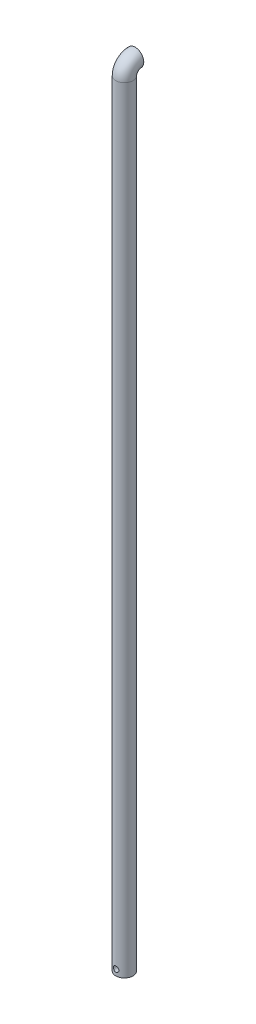
from build123d import *

# Parameters (mm, degrees)
SKETCH1_R               = 8
SKETCH1_R_2             = 3
SKETCH3_R               = 3
BOSS_EXTRUDE1_DEPTH     = 3
CUT_EXTRUDE2_DEPTH      = 731.265705073
CUT_EXTRUDE2_DEPTH_BACK = 731.265705073
SKETCH4_R               = 2.5


with BuildPart() as part:
    # Sweep1: sweep along a path in Sketch2
    with BuildLine(Plane(origin=(0, 0, 0), x_dir=(0, 0, -1), z_dir=(1, 0, 0))) as sweep1_path:
        Line((0, 0), (-0.05, 0))
        ThreePointArc((-0.05, 0), (-7.085712473, -2.914287527), (-10, -9.95))
        Line((-10, -9.95), (-10, -730))
    # Sketch1 → Sweep1 (sweep)
    with BuildSketch(Plane.XY):
        Circle(SKETCH1_R)
        Circle(SKETCH1_R_2, mode=Mode.SUBTRACT)
    sweep(path=sweep1_path.line)

    # Sketch3 → Boss-Extrude1 (add)
    with BuildSketch(Plane.XZ.offset(730)):
        with Locations(Location((0, 10, 0), (0, 0, 270))):
            Circle(SKETCH3_R)
    extrude(amount=-BOSS_EXTRUDE1_DEPTH)

    # Sketch4 → Cut-Extrude2 (cut, two sides: drawn at the far end of the back side and taken through both)
    with BuildSketch(Plane.XY.offset(-CUT_EXTRUDE2_DEPTH_BACK)):
        with Locations((0, -724.5)):
            Circle(SKETCH4_R)
    extrude(amount=CUT_EXTRUDE2_DEPTH + CUT_EXTRUDE2_DEPTH_BACK, mode=Mode.SUBTRACT)


solid = part.part
